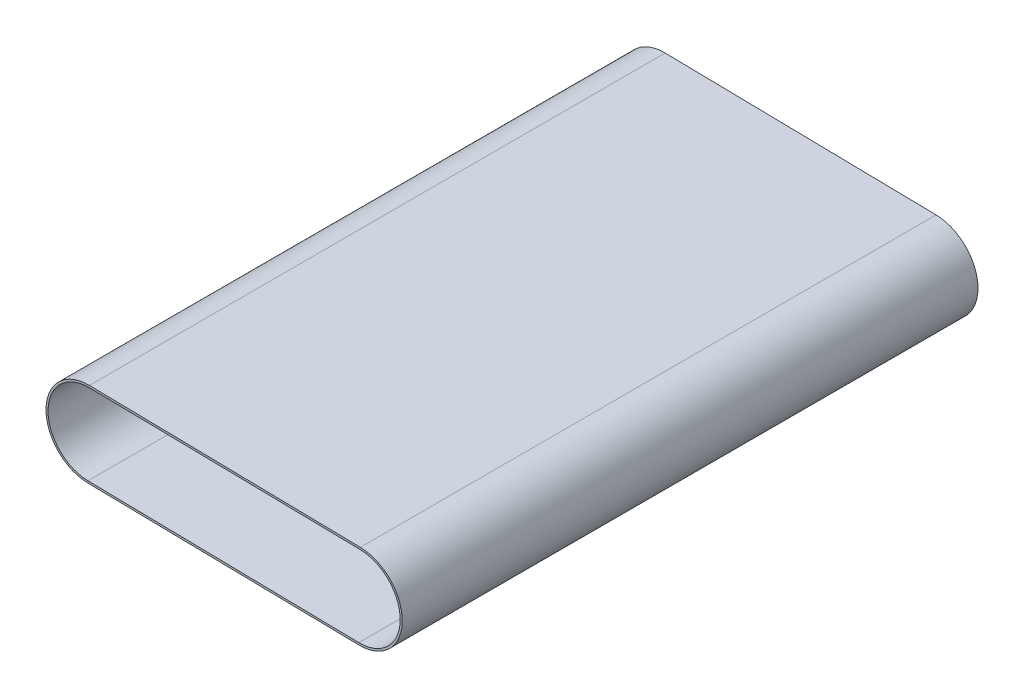
from build123d import *

# Parameters (mm, degrees)
EXTRUDE_1_DEPTH = 850


with BuildPart() as part:
    # 草图1 → 凸台-拉伸1 (new body)
    with BuildSketch(Plane(origin=(0, 0, 425), x_dir=(-1, 0, 0), z_dir=(0, 0, -1))):
        with BuildLine():
            Line((-601.038579668, 1587.00944222), (-201.099501606, 1593.990404795))
            ThreePointArc((-201.099501606, 1593.990404795), (-137.009595205, 1532.099501606), (-198.900498394, 1468.009595205))
            Line((-198.900498394, 1468.009595205), (-598.839576457, 1461.02863263))
            ThreePointArc((-598.839576457, 1461.02863263), (-662.929482857, 1522.91953582), (-601.038579668, 1587.00944222))
        make_face()
        with BuildLine():
            Line((-600.986222449, 1584.009899134), (-201.047144386, 1590.990861709))
            ThreePointArc((-201.047144386, 1590.990861709), (-140.009138291, 1532.047144386), (-198.952855614, 1471.009138291))
            Line((-198.952855614, 1471.009138291), (-598.891933676, 1464.028175716))
            ThreePointArc((-598.891933676, 1464.028175716), (-659.929939772, 1522.971893039), (-600.986222449, 1584.009899134))
        make_face(mode=Mode.SUBTRACT)
    extrude(amount=EXTRUDE_1_DEPTH)


solid = part.part
